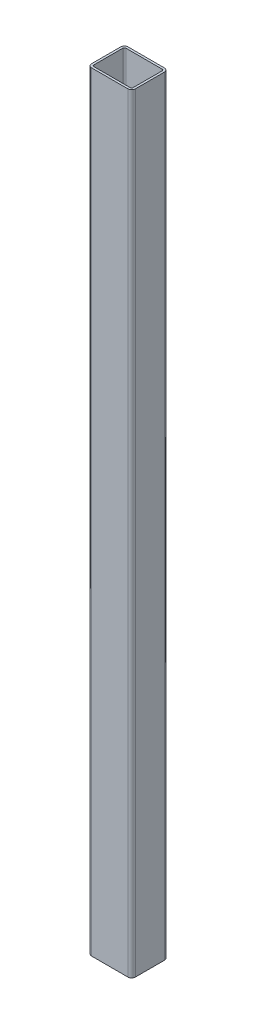
SolidWorks part; units mm, degrees
ref_plane "Front Plane" through (0, 0, 0) normal (0, 0, 1) x (1, 0, 0)
ref_plane "Top Plane" through (0, 0, 0) normal (0, 1, 0) x (1, 0, 0)
ref_plane "Right Plane" through (0, 0, 0) normal (1, 0, 0) x (0, 0, -1)
other "Configuration Table"
sketch "Sketch1" plane through (0, 0, 0) normal (0, 1, 0) x (1, 0, 0)
  line L1 (-50, 50) -> (50, 50)
  line L2 (-60, 40) -> (-60, -40)
  line L3 (-50, -50) -> (50, -50)
  line L4 (60, 40) -> (60, -40)
  line L5 (-60, 50) -> (60, -50) construction
  line L6 (-60, -50) -> (60, 50) construction
  arc A0 (50, 50) -> (60, 40) centre (50, 40) cw
  arc A1 (50, -50) -> (60, -40) centre (50, -40) ccw
  arc A2 (-60, -40) -> (-50, -50) centre (-50, -40) ccw
  arc A3 (-50, 50) -> (-60, 40) centre (-50, 40) ccw
  point P0 (0, 0)
  dimension "D3" = 10
  dimension "D1" = 120
  dimension "D2" = 100
extrude "Extrude-Thin1" add sketch "Sketch1" along normal mid plane 2114 thin
